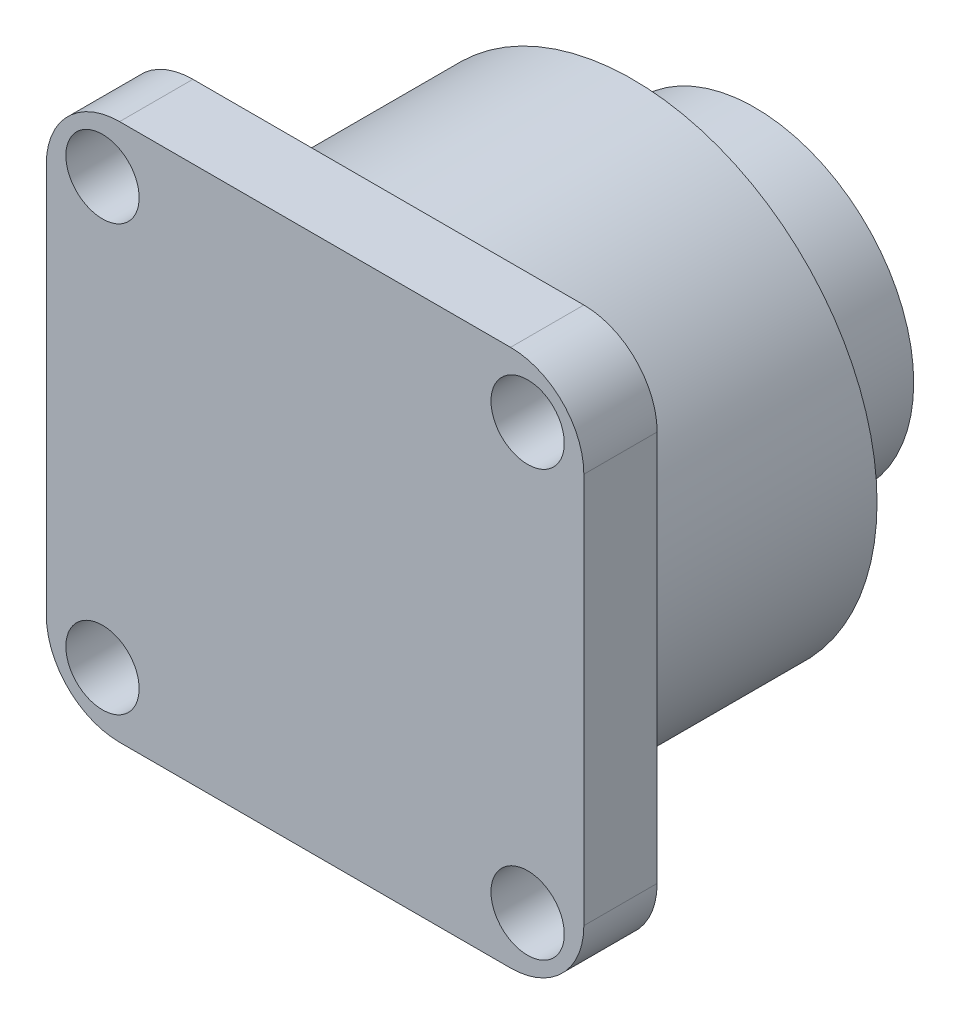
SolidWorks part; units mm, degrees
ref_plane "Front Plane" through (0, 0, 0) normal (0, 0, 1) x (1, 0, 0)
ref_plane "Top Plane" through (0, 0, 0) normal (0, 1, 0) x (1, 0, 0)
ref_plane "Right Plane" through (0, 0, 0) normal (1, 0, 0) x (0, 0, -1)
sketch "Sketch1" plane through (0, 0, 0) normal (0, 0, 1) x (1, 0, 0)
  circle A0 centre (-148.7461, 0) radius 6.5
  circle A1 centre (-148.7461, 0) radius 3
extrude "Boss-Extrude1" add sketch "Sketch1" along normal blind 5 contours A0
sketch "Sketch2" plane through (0, 0, 5) normal (0, 0, 1) x (1, 0, 0)
  circle A0 centre (-148.7461, 0) radius 10
extrude "Boss-Extrude2" add sketch "Sketch2" along normal blind 10
sketch "Sketch3" plane through (0, 0, 15) normal (0, 0, 1) x (1, 0, 0)
  line L1 (-159.7461, -11) -> (-137.7461, -11)
  line L2 (-159.7461, -11) -> (-159.7461, 11)
  line L3 (-159.7461, 11) -> (-137.7461, 11)
  line L4 (-137.7461, -11) -> (-137.7461, 11)
  line L5 (-159.7461, -11) -> (-137.7461, 11) construction
  line L6 (-159.7461, 11) -> (-137.7461, -11) construction
  point P0 (-148.7461, 0)
extrude "Boss-Extrude3" add sketch "Sketch3" along normal blind 3
fillet "Fillet1" radius 3 4 edges at (-137.7461, 11, 16.5) (-159.7461, -11, 16.5) (-137.7461, -11, 16.5) (-159.7461, 11, 16.5)
sketch "Sketch4" plane through (0, 0, 15) normal (0, 0, -1) x (-1, 0, 0)
  line L0 (140.7461, 11) -> (156.7461, 11) construction
  line L1 (159.7461, 8) -> (159.7461, -8) construction
  circle A0 centre (157.4461, 8.7) radius 1.5
  circle A1 centre (157.4461, -8.7) radius 1.5
  circle A2 centre (140.0461, -8.7) radius 1.5
  circle A3 centre (140.0461, 8.7) radius 1.5
  point P15 (148.7461, 0)
  dimension "D1" = 2.3
  dimension "D2" = 2.3
  dimension "D3" = 4
extrude "Cut-Extrude1" cut sketch "Sketch4" against normal blind 3
